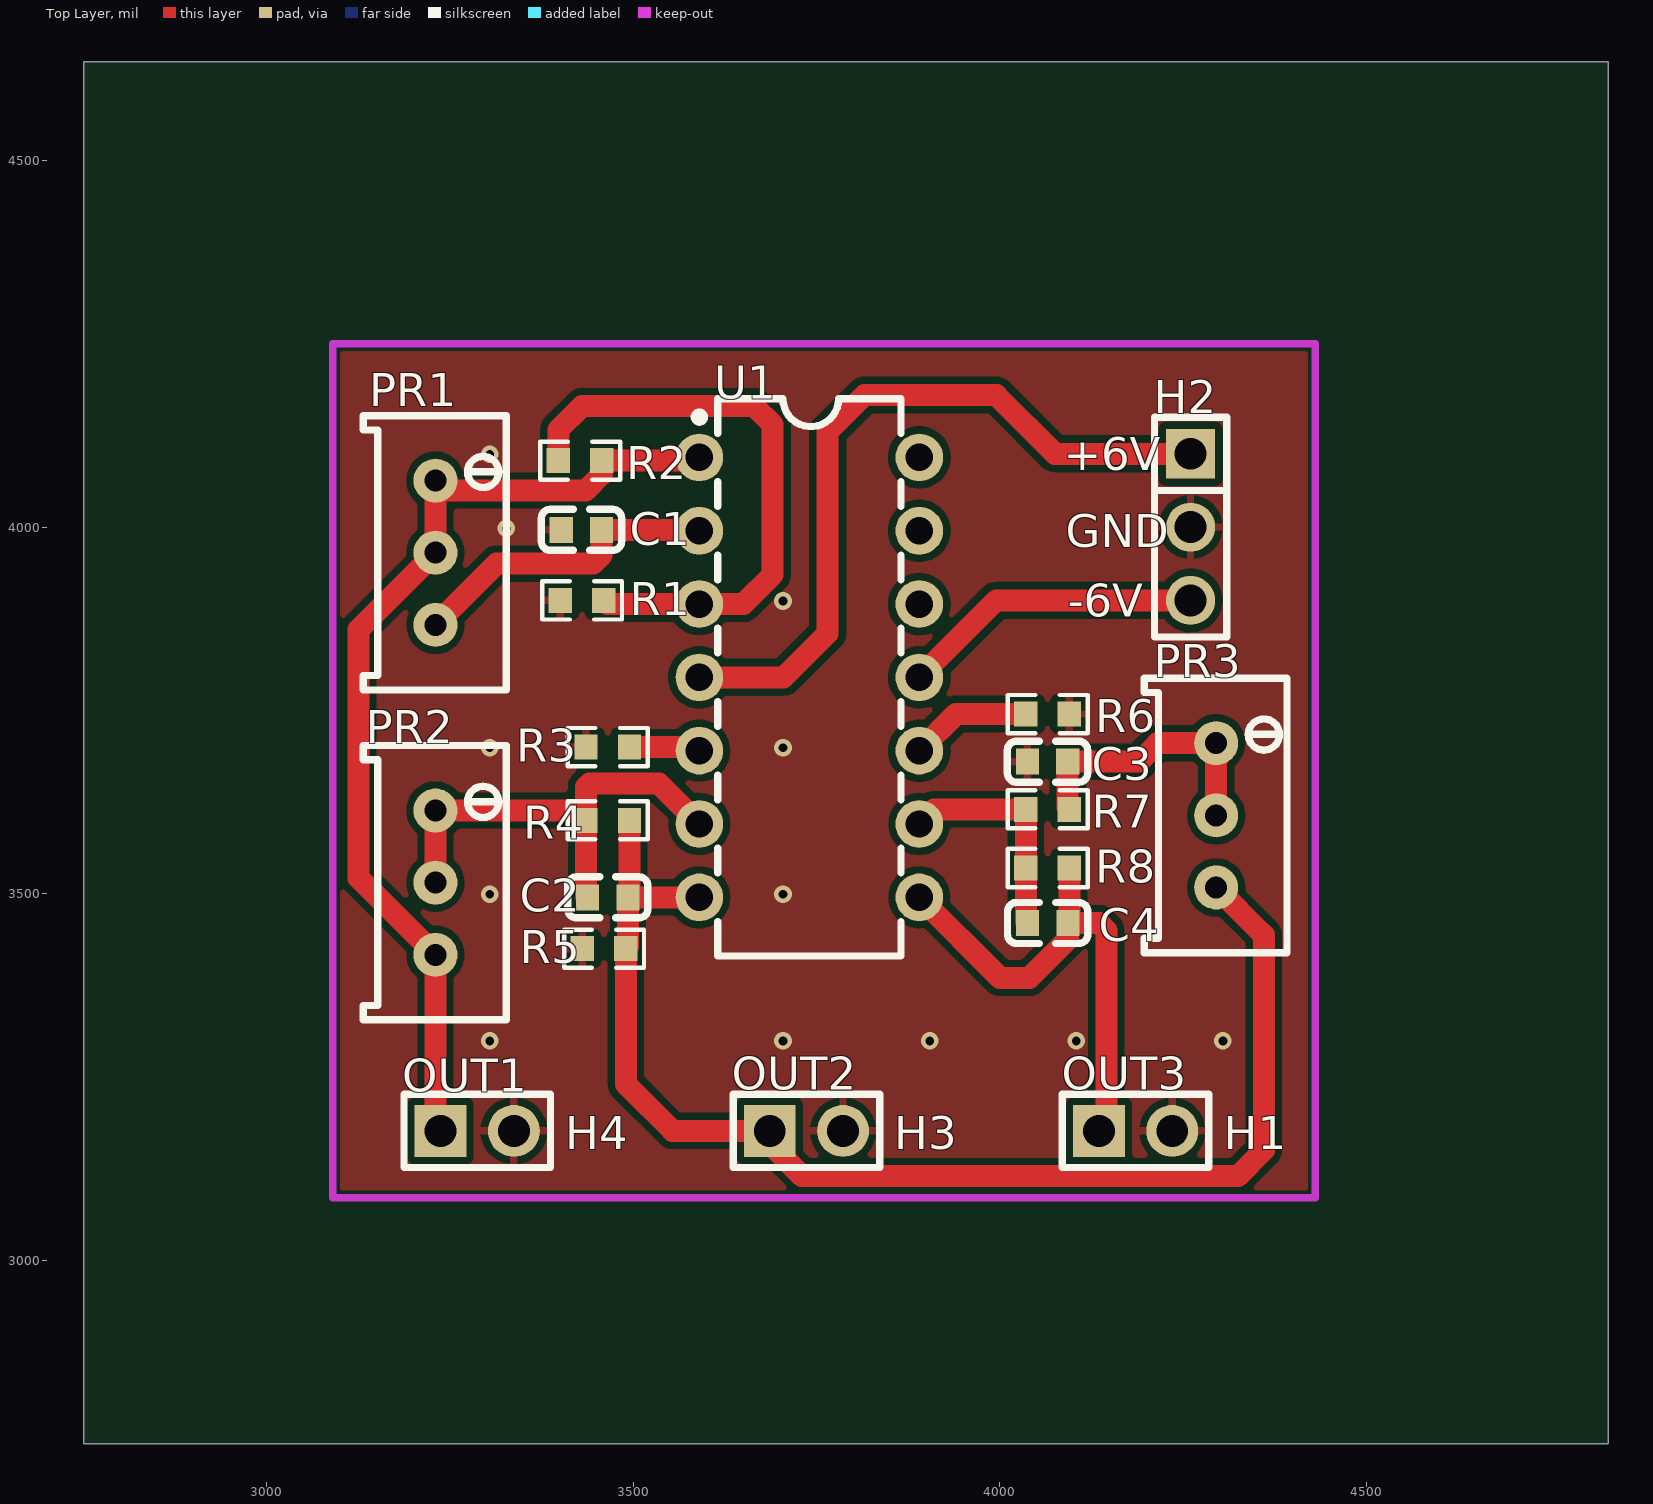
[diagram p0: Top Layer view]
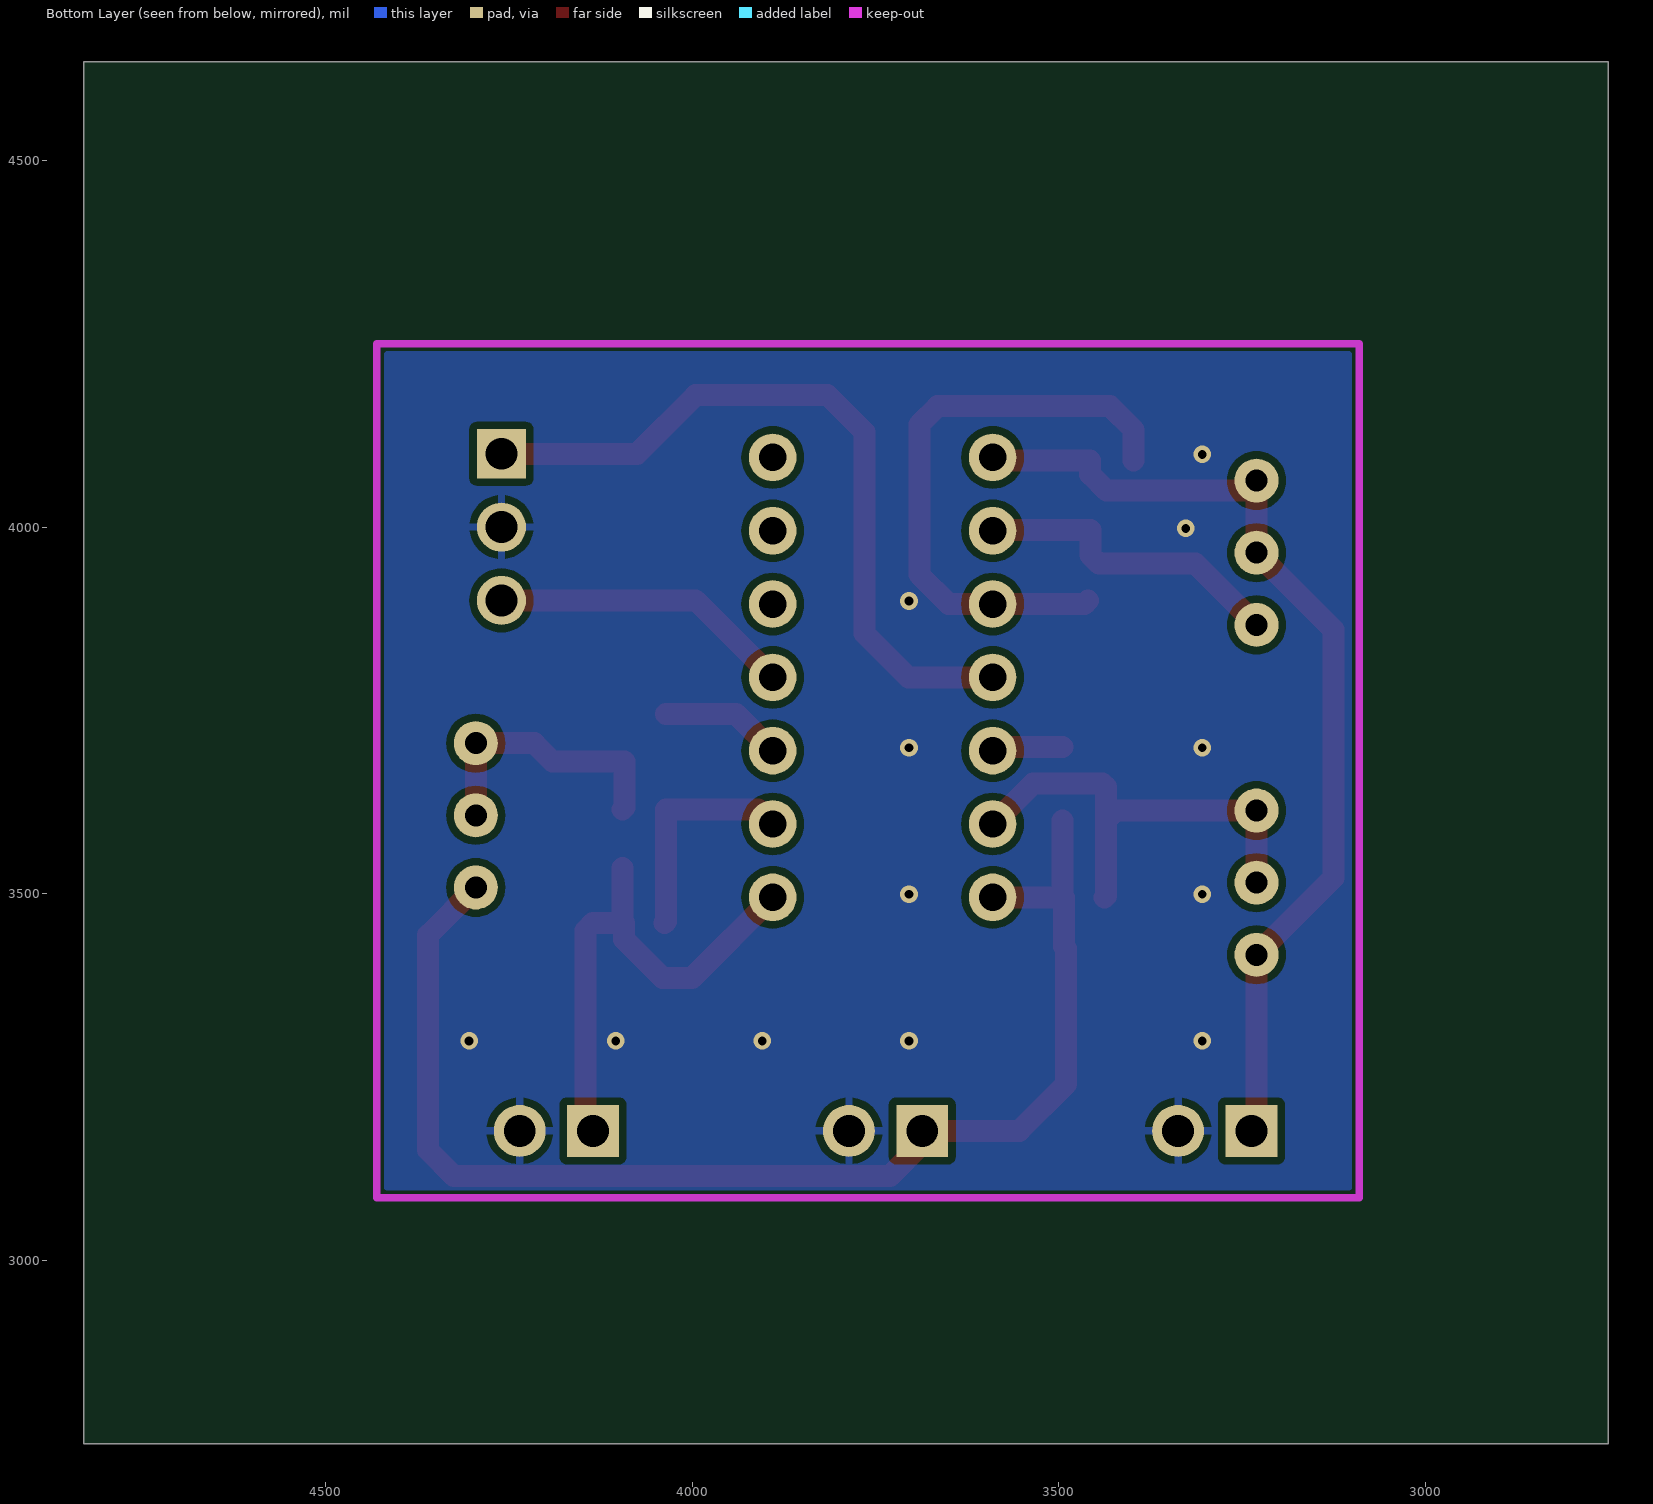
[diagram p1: Bottom Layer view, seen from below]
# Altium PCB MISC52110.pcbdoc
Units mil, origin at the board's own origin, x right, y up, seen from the top; angles counter-clockwise.
Board outline 2080 x 1885 mil, 2 copper layers (Top Layer, Bottom Layer), stack 62.206 mil thick; 20 components, 13 nets, 56 pads, 12 vias.

## Layer stack, top to bottom
Top Solder Mask Layer: solder mask 0.394, Dk 3.3
Top Layer: signal copper 1.379
Dielectric1: surface 59.449, FR4, Dk 4.5
Bottom Layer: signal copper 1.378
Bottom Solder Mask Layer: solder mask 0.394, Dk 3.3

## Board outline
4830,2750 2750,2750 2750,4635 4830,4635

## Design rules (kind name [scope] priority, off if disabled: settings)
BoardOutlineClearance copperThickness2oz_1 [All] p2 off: genericclearance=7.99 ignorepadtopadclearanceinfootprint=FALSE except(0: Arc-SplitContinuation Track-SplitContinuation SMDPad-SplitContinuation THPad-SplitContinuation Via-SplitContinuation Fill-SplitContinuation Region-SplitContinuation Poly-SplitContinuation Text-SplitContinuation Hole-SplitContinuation; 5.98: Arc-CutoutEdge SMDPad-CutoutEdge THPad-CutoutEdge Via-CutoutEdge Fill-CutoutEdge Region-CutoutEdge Text-CutoutEdge; 6.93: Hole-OutlineEdge Hole-CutoutEdge; 10: Poly-OutlineEdge Poly-CutoutEdge; 11.81: Arc-OutlineEdge Track-OutlineEdge SMDPad-OutlineEdge THPad-OutlineEdge Via-OutlineEdge Fill-OutlineEdge Region-OutlineEdge Text-OutlineEdge Track-CutoutEdge)
BoardOutlineClearance copperThickness1oz_1 [All] p4: genericclearance=4.02 ignorepadtopadclearanceinfootprint=FALSE except(0: Arc-SplitContinuation Track-SplitContinuation SMDPad-SplitContinuation THPad-SplitContinuation Via-SplitContinuation Fill-SplitContinuation Region-SplitContinuation Poly-SplitContinuation Text-SplitContinuation Hole-SplitContinuation; 6: SMDPad-CutoutEdge THPad-CutoutEdge Via-CutoutEdge Fill-CutoutEdge Region-CutoutEdge Text-CutoutEdge; 6.93: Hole-OutlineEdge Hole-CutoutEdge; 10: Poly-OutlineEdge Poly-CutoutEdge; 11.8: Arc-OutlineEdge Track-OutlineEdge SMDPad-OutlineEdge THPad-OutlineEdge Via-OutlineEdge Fill-OutlineEdge Region-OutlineEdge Text-OutlineEdge; 11.81: Arc-CutoutEdge Track-CutoutEdge)
Clearance copperThickness2oz [All] p1 off: gap=7.99 ignorepadtopadclearanceinfootprint=FALSE except(5.98: SMDPad-Track SMDPad-SMDPad THPad-Track SMDPad-THPad THPad-THPad Track-Via SMDPad-Via THPad-Via Via-Via Fill-Track Region-Track Fill-SMDPad Region-SMDPad Fill-THPad Region-THPad Fill-Via Region-Via Fill-Fill Fill-Region Region-Region Arc-Track Arc-SMDPad Arc-THPad Arc-Via Fill-Arc Region-Arc Arc-Arc Text-Track SMDPad-Text Text-THPad Text-Via Fill-Text Region-Text Arc-Text Text-Text; 6.93: Hole-Track Hole-SMDPad Hole-THPad Hole-Via Fill-Hole Region-Hole Hole-Arc Hole-Text; 10: Poly-Track Poly-SMDPad Poly-THPad Poly-Via Poly-Fill Poly-Region Poly-Poly Poly-Arc Poly-Text Poly-Hole)
Clearance copperThickness1oz [All] p3: gap=4.02 ignorepadtopadclearanceinfootprint=FALSE except(5.98: SMDPad-Track SMDPad-SMDPad THPad-Track SMDPad-THPad THPad-THPad Track-Via SMDPad-Via THPad-Via Via-Via Fill-Track Region-Track Fill-SMDPad Region-SMDPad Fill-THPad Region-THPad Fill-Via Region-Via Fill-Fill Fill-Region Region-Region; 6: Arc-Track Arc-SMDPad Arc-THPad Arc-Via Fill-Arc Region-Arc Arc-Arc Text-Track SMDPad-Text Text-THPad Text-Via Fill-Text Region-Text Arc-Text Text-Text; 6.93: Hole-Track Hole-SMDPad Hole-THPad Hole-Via Fill-Hole Region-Hole Hole-Arc Hole-Text; 10: Poly-Track Poly-SMDPad Poly-THPad Poly-Via Poly-Fill Poly-Region Poly-Poly Poly-Arc Poly-Text Poly-Hole)
DiffPairsRouting differentialPair [All] p1: maxlimit=6 minlimit=6 mostfreqgap=6 toplayer_minwidth=5 toplayer_prefwidth=10 toplayer_maxwidth=100 toplayer_mingap=6 toplayer_prefgap=6 toplayer_maxgap=6 bottomlayer_minwidth=5 bottomlayer_prefwidth=10 bottomlayer_maxwidth=100 bottomlayer_mingap=6 bottomlayer_prefgap=6 bottomlayer_maxgap=6 maxuncoupledlength=10
HoleToHoleClearance otherClearance [All] p1: gap=11.81 allowstackedmicrovias=TRUE
Length netLength [All] p1: minlimit=0 maxlimit=0
MatchedLengths netLengthTolerance [All] p1: tolerance=1000
PasteMaskExpansion pasteMaskExpansion [All] p1: expansion=0
PlaneConnect innerPlane [All] p1: planeconnectstyle=Relief reliefexpansion=20 reliefentries=4 reliefconductorwidth=10 reliefairgap=10
PolygonConnect copperRegion [(InNet('GND'))] p1: connectstyle=Relief reliefconductorwidth=10 reliefentries=4 polygonreliefangle="90 Angle" airgapwidth=10 via.connectstyle=Relief via.reliefconductorwidth=10 via.reliefentries=4 via.polygonreliefangle="90 Angle" via.airgapwidth=10
RoutingVias viaSize [All] p1: holewidth=12.01 width=24.02 viastyle="Through Hole" minholewidth=11.81 minwidth=19.68 maxholewidth=248.03 maxwidth=393.7
SolderMaskExpansion solderMaskExpansion [IsVia] p1: expansion=-1000 istentingtop=TRUE
SolderMaskExpansion solderMaskExpansion [All] p2: expansion=2 istentingtop=FALSE
Width copperThickness2oz_2 [All] p1 off: maxlimit=100 minlimit=8 preferedwidth=10
Width copperThickness1oz_2 [All] p2: maxlimit=100 minlimit=5 preferedwidth=10

## Components (designator, comment, footprint, x,y, rotation, side; value= is the part's Value field where it differs from the comment)
C1 "30nF" C0603 3429.22,3996.21 r0 top
C2 "100nF" C0603 3465,3495 r0 top
C3 "100nF" C0603 4064.88,3680 r0 top
C4 "100nF" C0603 4065,3460 r0 top
H1 "" HDR-TH_2P-P2.54-V-M-1 4185,3176.4 r0 top
H2 "" HDR-TH_3P-P2.54-V-M 4260,4000 r270 top
H3 "" HDR-TH_2P-P2.54-V-M-1 3736,3176.4 r0 top
H4 "" HDR-TH_2P-P2.54-V-M-1 3287,3176.4 r0 top
PR1 "10kΩ" R_3296 3235,3965 r270 top
PR2 "20kΩ" R_3296 3235,3515 r270 top
PR3 "200kΩ" R_3296 4300,3606.8 r270 top
R1 "10K" R0603 3430,3900 r0 top
R2 "3.9kΩ" R0603 3427.28,4090.63 r180 top
R3 "100K" R0603 3465,3700 r0 top
R4 "300K" R0603 3465,3600 r0 top
R5 "620" R0603 3460,3425 r0 top
R6 "10K" R0603 4065,3745 r180 top
R7 "20K" R0603 4065,3615 r180 top
R8 "24K" R0603 4065,3535 r0 top
U1 "LM324N/PB" PDIP-14_L19.2-W6.6-P2.54-LS7.6-BL 3740,3795 r270 top

## Footprints (in the part's own frame and the unit in brackets; to place one, negate y for a bottom-side part, rotate by r counter-clockwise, add the part's x,y. Pads: shape width x height; smd on the part's side, far side on the other; paste and mask are expansions set on the pad)
C0603 [mm]
  rect 0.8x0.9 smd: 1(-0.7,0) 2(0.7,0)
  silkscreen extent -1.39,-0.71 1.39,0.71
HDR-TH_2P-P2.54-V-M-1 [mm]
  rect 1.8x1.8 hole 1.1: 1(-1.27,0)
  round 1.8 hole 1.1: 2(1.27,0)
  silkscreen extent -2.54,-1.27 2.54,1.27
HDR-TH_3P-P2.54-V-M [mm]
  rect 1.7x1.7 hole 1.1: 1(-2.54,0)
  round 1.7 hole 1.1: 2(0,0) 3(2.54,0)
  silkscreen extent -3.81,-1.25 3.81,1.25
PDIP-14_L19.2-W6.6-P2.54-LS7.6-BL [mm]
  round 1.65 hole 0.95: 1(-7.62,-3.81) 2(-5.08,-3.81) 3(-2.54,-3.81) 4(0,-3.81) 5(2.54,-3.81) 6(5.08,-3.81) 7(7.62,-3.81) 8(7.62,3.81) 9(5.08,3.81) 10(2.54,3.81) 11(0,3.81) 12(-2.54,3.81) 13(-5.08,3.81) 14(-7.62,3.81)
  silkscreen extent -9.65,-3.96 9.65,3.17
R0603 [mil]
  rect 31.75x34.02 smd paste-3937.01 mask+2: 1(-29.66,0) 2(29.66,0)
  silkscreen extent -55,-26 55,26
R_3296 [mil]
  round 60 hole 30 paste+0 mask+2: 1(-98.4,-5) 2(0,-5) 3(98.4,-5)
  silkscreen extent -187,-103 187,92

## Via types
v1: diameter 24.02, hole 12, Top Layer to Bottom Layer, 12 vias

## Nets (pads, with @x,y where several pads share a name; then routed paths per layer and width w, separated by ;. In a path a pad name is that pad's centre, name@x,y a point inside that pad or via, vN(x,y) a via of type N, cw(c..) or ccw(c..) an arc to the next point about the centre after c; other vN are vias at no path point)
6V: H2.1 U1.4 | length 1023.7
  Top Layer w30: U1.4 3705,3795 3765,3855 3765,4130 3815,4180 3995,4180 4075,4100 H2.1
$1N1: R1.2 R2.2 U1.3 | length 812.1
  Top Layer w30: R2.2 3397.62,4132.62 3430,4165 3665,4165 3690,4140 3690,3935 3650,3895 U1.3 3464.66,3895 R1.2
$1N4: C1.2 PR1.3 U1.2 | length 434.4
  Top Layer w30: PR1.3 3313.4,3950 3445,3950 3456.78,3961.78 C1.2 3588.8,3996.21 U1.2
$1N8: H4.1 PR1.1 PR1.2 PR2.3 R2.1 U1.1 | length 1372
  Top Layer w30: H4.1 3230,3183.4 PR2.3 3125,3521.6 3125,3860 PR1.2 PR1.1 3243.4,4050 3435,4050 3456.94,4071.94 R2.1 3585.63,4090.63 U1.1
$1N9: R3.2 U1.5 | length 97.4
  Top Layer w30: R3.2 3585.01,3700 U1.5
$1N11: C2.2 H3.1 PR3.3 R4.2 R5.2 U1.7 | length 1791.4
  Top Layer w30: R4.2 3494.66,3497.1 C2.2 ; U1.7 C2.2 ; PR3.3 4360,3443.4 4360,3150 4325,3115 3730,3115 3686,3159 H3.1 3553.6,3176.4 3489.66,3240.34 R5.2 3492.56,3427.9 C2.2
$1N12: C2.1 PR2.1 PR2.2 R4.1 U1.6 | length 639.9
  Top Layer w30: PR2.2 PR2.1 3421.94,3613.4 R4.1 ; C2.1 3435.34,3497.1 R4.1 ; U1.6 3535.01,3650 3440,3650 3435.34,3645.34 R4.1
$1N17: R6.2 U1.10 | length 166
  Top Layer w30: U1.10 3940,3745 R6.2
$1N19: C4.1 R7.2 R8.1 U1.9 | length 309.5
  Top Layer w30: U1.9 3910,3615 R7.2 R8.1 4035.34,3462.1 C4.1
$1N20: C3.2 PR3.1 PR3.2 R7.1 | length 377.3
  Top Layer w30: R7.1 4092.44,3617.22 C3.2 4190,3680 4215.2,3705.2 PR3.1 PR3.2
$1N22: C4.2 H1.1 R8.2 U1.8 | length 702.5
  Top Layer w30: U1.8 4000.01,3385 4040,3385 4092.56,3437.56 C4.2 ; R8.2 4094.66,3462.1 C4.2 ; H1.1 4145,3186.4 4145,3450 4135,3460 C4.2
-6V: H2.3 U1.11 | length 413.5
  Top Layer w30: U1.11 3995,3900 H2.3
GND: C1.1 C3.1 H1.2 H2.2 H3.2 H4.2 R1.1 R3.1 R5.1 R6.1
  other v1: 3304.1,3299.1 3704.1,3299.1 3904.1,3299.1 4104.1,3299.1 4304.1,3299.1 3304.1,3499.1 3704.1,3499.1 3304.1,3699.1 3704.1,3699.1 3704.1,3899.1 3326.5,3998.18 3304.1,4099.1
pads on no net: U1.12 U1.13 U1.14

## Polygon pours and split planes (outlines as drawn)
GND on Top Layer (solid, remove dead copper, pour order 0): 3000,4385 3000,3055 4460,3055 4460,4385
GND on Bottom Layer (solid, remove dead copper, pour order 2): 3010,4370 3010,3000 4580,3000 4580,4370

## Keep-outs
Board Outline Layer:
  lines w10: 3090,3085 3090,4250 4430,4250 4430,3085 3090,3085

## Silkscreen, mask and mechanical layers (free items; w line width, h text height)
Top Silkscreen Layer:
  text "+6V" at 4086.99,4077.5 h45
  text "GND" at 4089.4,3972.5 h45
  text "-6V" at 4092.26,3877.5 h45
  text "OUT2" at 3634.4,3232.5 h45
  text "OUT3" at 4084.4,3232.5 h45
  text "OUT1" at 3185,3230 h45